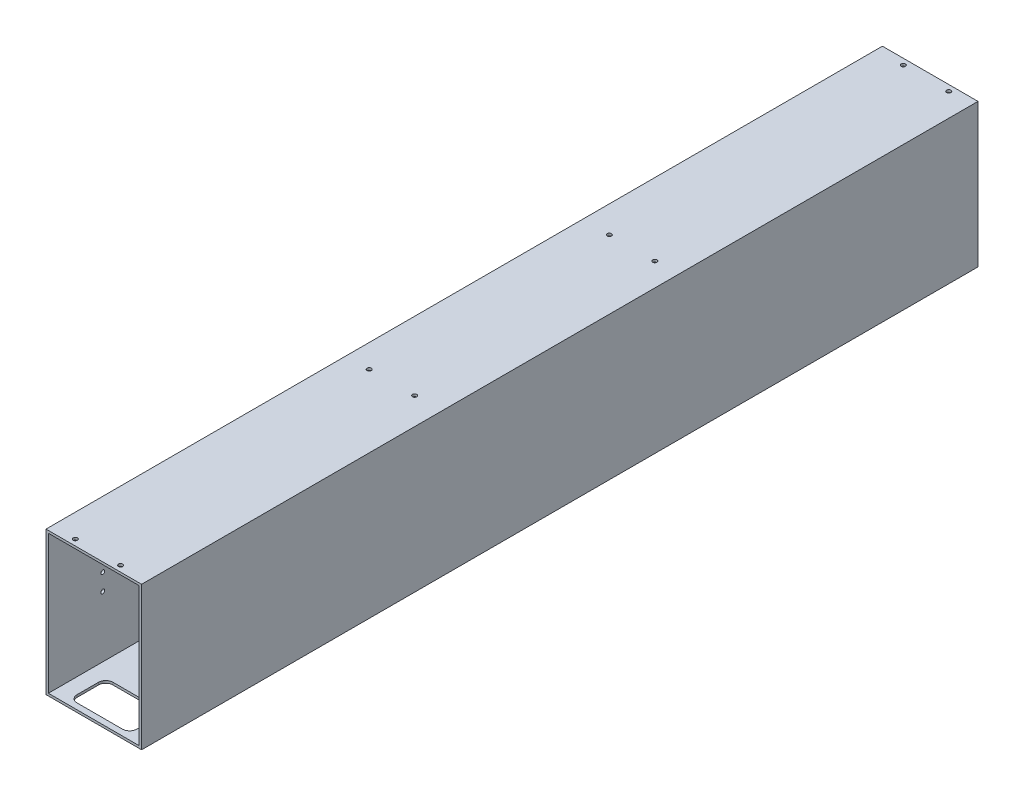
from build123d import *

# Parameters (mm, degrees)
SKETCH_1_W             = 80
SKETCH_1_H             = 120
SKETCH_1_W_2           = 76
SKETCH_1_H_2           = 116
EXTRUDE_1_DEPTH        = 350
CUT_EXTRUDE_2_REACH    = 366.005
SKETCH_4_R             = 25
HOLE_WIZARD_M4_1_D     = 3.3
HOLE_WIZARD_M4_1_DEPTH = 2
HOLE_WIZARD_M3_1_D     = 3.6
HOLE_WIZARD_M3_1_DEPTH = 2
CUT_EXTRUDE_3_REACH    = 374.156
SKETCH_16_W            = 50
SKETCH_16_H            = 30
SKETCH_16_W_2          = 60
SKETCH_16_H_2          = 100
FILLET_1_R             = 6


with BuildPart() as part:
    # 草图1 → 拉伸-薄壁1 (new, symmetric)
    with BuildSketch(Plane.XY):
        Rectangle(SKETCH_1_W, SKETCH_1_H)
        Rectangle(SKETCH_1_W_2, SKETCH_1_H_2, mode=Mode.SUBTRACT)
    extrude(amount=EXTRUDE_1_DEPTH, both=True)

    # 草图4 → 切除-拉伸2 (cut, up to next)
    with BuildSketch(Plane.ZY.offset(40), mode=Mode.PRIVATE) as cut_extrude_2_sk1:
        with Locations((0, -20)):
            Circle(SKETCH_4_R)
    cut_extrude_2_tool1 = extrude(cut_extrude_2_sk1.sketch, amount=-CUT_EXTRUDE_2_REACH, mode=Mode.PRIVATE) & part.part
    add(cut_extrude_2_tool1.solids().sort_by_distance((-40, -20, 0))[0], mode=Mode.SUBTRACT)

    # Hole Wizard M4 _1
    with Locations(Plane.ZY.offset(40)):
        with Locations((304.5, 29), (304.5, 15), (304.5, 7), (304.5, -7), (-304.5, -7), (-304.5, 7), (-304.5, 15), (-304.5, 29)):
            Hole(HOLE_WIZARD_M4_1_D / 2, depth=HOLE_WIZARD_M4_1_DEPTH)

    # M3 间隙孔1
    with Locations(Plane(origin=(0, 60, 0), x_dir=(1, 0, 0), z_dir=(0, 1, 0))):
        with Locations((-17.5, 345), (20.5, 345), (20.5, 99), (-17.5, 99), (-20.5, -345), (17.5, -345), (-20.5, -99), (17.5, -99)):
            Hole(HOLE_WIZARD_M3_1_D / 2, depth=HOLE_WIZARD_M3_1_DEPTH)

    # 草图16 → 切除-拉伸3 (cut, up to next)
    with BuildSketch(Plane.XZ.offset(60), mode=Mode.PRIVATE) as cut_extrude_3_sk1:
        with Locations((0, 330)):
            Rectangle(SKETCH_16_W, SKETCH_16_H)
    cut_extrude_3_tool1 = extrude(cut_extrude_3_sk1.sketch, amount=-CUT_EXTRUDE_3_REACH, mode=Mode.PRIVATE) & part.part
    # 草图16 → 切除-拉伸3 (cut, up to next)
    with BuildSketch(Plane.XZ.offset(60), mode=Mode.PRIVATE) as cut_extrude_3_sk2:
        with Locations((0, 145)):
            Rectangle(SKETCH_16_W_2, SKETCH_16_H_2)
    cut_extrude_3_tool2 = extrude(cut_extrude_3_sk2.sketch, amount=-CUT_EXTRUDE_3_REACH, mode=Mode.PRIVATE) & part.part
    # 草图16 → 切除-拉伸3 (cut, up to next)
    with BuildSketch(Plane.XZ.offset(60), mode=Mode.PRIVATE) as cut_extrude_3_sk3:
        with Locations((0, -145)):
            Rectangle(SKETCH_16_W_2, SKETCH_16_H_2)
    cut_extrude_3_tool3 = extrude(cut_extrude_3_sk3.sketch, amount=-CUT_EXTRUDE_3_REACH, mode=Mode.PRIVATE) & part.part
    # 草图16 → 切除-拉伸3 (cut, up to next)
    with BuildSketch(Plane.XZ.offset(60), mode=Mode.PRIVATE) as cut_extrude_3_sk4:
        with Locations((0, -330)):
            Rectangle(SKETCH_16_W, SKETCH_16_H)
    cut_extrude_3_tool4 = extrude(cut_extrude_3_sk4.sketch, amount=-CUT_EXTRUDE_3_REACH, mode=Mode.PRIVATE) & part.part
    add(cut_extrude_3_tool1.solids().sort_by_distance((0, -60, 330))[0], mode=Mode.SUBTRACT)
    add(cut_extrude_3_tool2.solids().sort_by_distance((0, -60, 145))[0], mode=Mode.SUBTRACT)
    add(cut_extrude_3_tool3.solids().sort_by_distance((0, -60, -145))[0], mode=Mode.SUBTRACT)
    add(cut_extrude_3_tool4.solids().sort_by_distance((0, -60, -330))[0], mode=Mode.SUBTRACT)

    # 圆角1
    fillet_1_edges = [part.edges().sort_by_distance(p)[0] for p in [
        (25, -59, 315),
        (25, -59, 345),
        (-25, -59, 345),
        (-25, -59, 315),
        (30, -59, 95),
        (30, -59, 195),
        (-30, -59, 195),
        (-30, -59, 95),
        (30, -59, -95),
        (-30, -59, -95),
        (-30, -59, -195),
        (30, -59, -195),
        (25, -59, -315),
        (-25, -59, -315),
        (-25, -59, -345),
        (25, -59, -345),
    ]]
    fillet(fillet_1_edges, radius=FILLET_1_R)


solid = part.part
